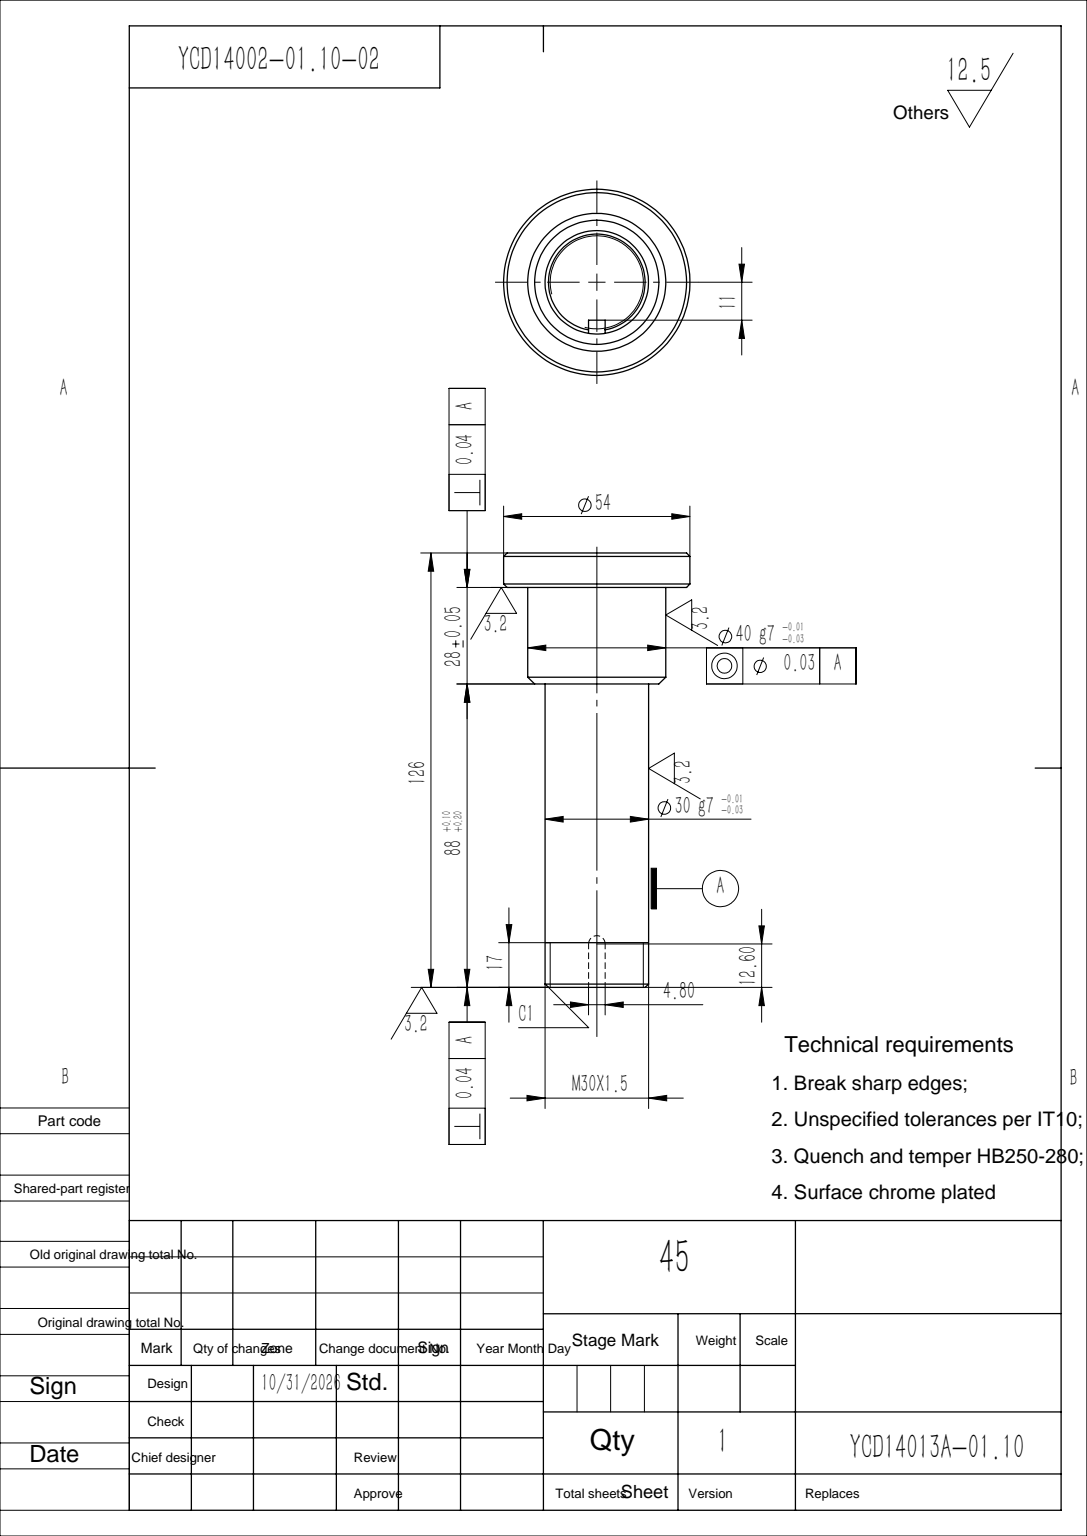
from build123d import *

# Parameters (mm, degrees)
SKETCH1_R           = 20
BOSS_EXTRUDE1_DEPTH = 28
SKETCH2_R           = 27
BOSS_EXTRUDE2_DEPTH = 10
SKETCH3_R           = 15
BOSS_EXTRUDE3_DEPTH = 88
CHAMFER1_SIZE       = 1
CHAMFER2_SIZE       = 2
CUT_EXTRUDE2_START  = -11
CUT_EXTRUDE2_DEPTH  = 11


with BuildPart() as part:
    # Sketch1 → Boss-Extrude1 (new body)
    with BuildSketch(Plane(origin=(0, 0, 0), x_dir=(1, 0, 0), z_dir=(0, 1, 0))):
        with Locations(Location((0, 0, 0), (0, 0, 270))):
            Circle(SKETCH1_R)
    extrude(amount=BOSS_EXTRUDE1_DEPTH)

    # Sketch2 → Boss-Extrude2 (add)
    with BuildSketch(Plane(origin=(0, 28, 0), x_dir=(1, 0, 0), z_dir=(0, 1, 0))):
        with Locations(Location((0, 0, 0), (0, 0, 270))):
            Circle(SKETCH2_R)
    extrude(amount=BOSS_EXTRUDE2_DEPTH)

    # Sketch3 → Boss-Extrude3 (add)
    with BuildSketch(Plane.XZ):
        with Locations(Location((0, 0, 0), (0, 0, 90))):
            Circle(SKETCH3_R)
    extrude(amount=BOSS_EXTRUDE3_DEPTH)

    # Chamfer1
    chamfer1_edges = [part.edges().sort_by_distance(p)[0] for p in [
        (0, -88, -15),
        (0, 28, -27),
        (0, 38, -27),
    ]]
    chamfer(chamfer1_edges, length=CHAMFER1_SIZE)

    # Chamfer2
    chamfer2_edges = [part.edges().sort_by_distance(p)[0] for p in [
        (0, 0, -20),
    ]]
    chamfer(chamfer2_edges, length=CHAMFER2_SIZE)

    # Sketch5 → Cut-Extrude2 (cut)
    with BuildSketch(Plane.XY.offset(CUT_EXTRUDE2_START)):
        with BuildLine():
            Line((-2.4, -100.6), (2.4, -100.6))
            Line((2.4, -100.6), (2.4, -75.4))
            ThreePointArc((2.4, -75.4), (0, -73), (-2.4, -75.4))
            Line((-2.4, -75.4), (-2.4, -100.6))
        make_face()
    extrude(amount=-CUT_EXTRUDE2_DEPTH, mode=Mode.SUBTRACT)


solid = part.part
